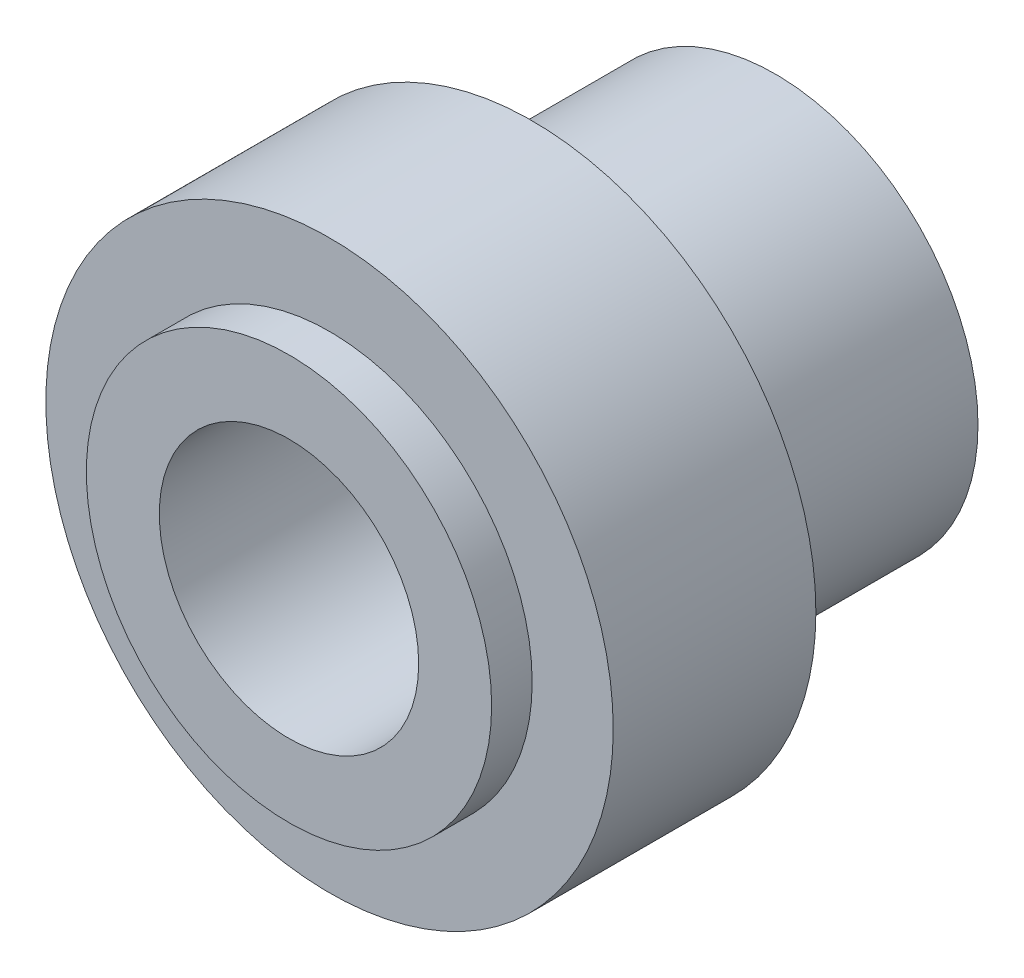
from build123d import *

# Parameters (mm, degrees)
SKETCH_1_R      = 5
SKETCH_1_R_2    = 3.2
EXTRUDE_1_DEPTH = 6
SKETCH_2_R      = 7
SKETCH_2_R_2    = 3.2
EXTRUDE_2_DEPTH = 5


with BuildPart() as part:
    # 草图1 → 凸台-拉伸1 (new, symmetric)
    with BuildSketch(Plane.XY):
        Circle(SKETCH_1_R)
        Circle(SKETCH_1_R_2, mode=Mode.SUBTRACT)
    extrude(amount=EXTRUDE_1_DEPTH, both=True)

    # 草图2 → 凸台-拉伸2 (add)
    with BuildSketch(Plane.XY):
        Circle(SKETCH_2_R)
        Circle(SKETCH_2_R_2, mode=Mode.SUBTRACT)
    extrude(amount=EXTRUDE_2_DEPTH)


solid = part.part
